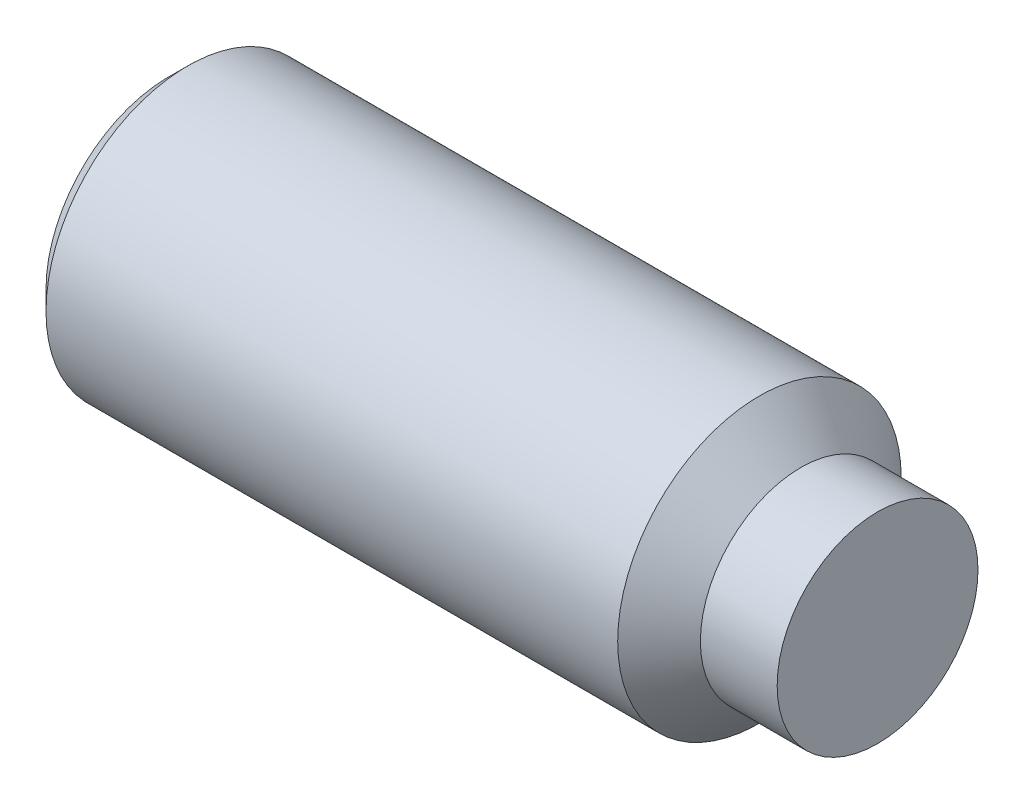
from build123d import *

# Parameters (mm, degrees)
CUT_EXTRUDE_1_DEPTH = 4.8


with BuildPart() as part:
    # 草图1 → Revolve 598 (revolve)
    with BuildSketch(Plane.XY, mode=Mode.PRIVATE) as revolve_598_sk:
        Polygon((0, 0), (30, 0), (30, 4.25), (26.75, 4.25), (25, 6), (0.804, 6), (0, 5.196), align=None)
    revolve(revolve_598_sk.sketch.rotate(Axis((-0.665465891, 0, 0), (1, 0, 0)), 90), axis=Axis((-0.665465891, 0, 0), (1, 0, 0)))

    # 草图2 → 切除-拉伸1 (cut)
    with BuildSketch(Plane.ZY):
        Polygon((3.43, 0), (1.715, 2.970467135), (-1.715, 2.970467135), (-3.43, 0), (-1.715, -2.970467135), (1.715, -2.970467135), align=None)
    extrude(amount=-CUT_EXTRUDE_1_DEPTH, mode=Mode.SUBTRACT)

    # 草图3 → 切除-旋转1 (revolve, cut)
    with BuildSketch(Plane.XY, mode=Mode.PRIVATE) as cut_revolve_1_sk:
        Polygon((4.8, 2.970467135), (6.515, 0), (4.8, 0), align=None)
    revolve(cut_revolve_1_sk.sketch.rotate(Axis((-0.262128326, 0, 0), (1, 0, 0)), 90), axis=Axis((-0.262128326, 0, 0), (1, 0, 0)), mode=Mode.SUBTRACT)


solid = part.part
